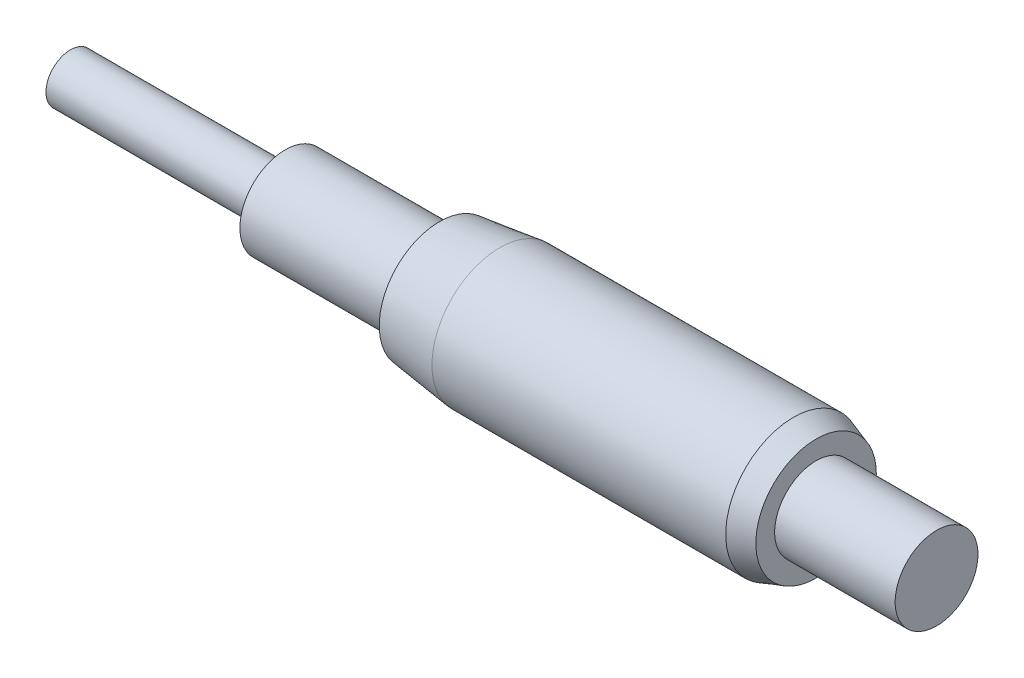
SolidWorks part; units mm, degrees
ref_plane "Front Plane" through (0, 0, 0) normal (0, 0, 1) x (1, 0, 0)
ref_plane "Top Plane" through (0, 0, 0) normal (0, 1, 0) x (1, 0, 0)
ref_plane "Right Plane" through (0, 0, 0) normal (1, 0, 0) x (0, 0, -1)
sketch "Sketch1" plane through (0, 0, 0) normal (0, 0, 1) x (1, 0, 0)
  line L0 (28.5, 3.25) -> (0, 3.25)
  line L1 (0, 3.25) -> (0, 0)
  line L2 (57, 9) -> (96, 9)
  line L3 (49, 8) -> (57, 9)
  line L4 (49, 6) -> (28.5, 6)
  line L5 (28.5, 6) -> (28.5, 3.25)
  line L7 (49, 8) -> (49, 6)
  line L8 (99, 5.5) -> (99, 8)
  line L9 (99, 8) -> (96, 9)
  line L10 (115, 0) -> (115, 5.5)
  line L11 (115, 5.5) -> (99, 5.5)
  line L12 (115, 0) -> (0, 0) construction
  line L13 (0, 0) -> (115, 0)
  dimension "D1" = 115
  dimension "D2" = 28.5
  dimension "D3" = 6
  dimension "D4" = 9
  dimension "D5" = 20.5
revolve "Revolve1" add sketch "Sketch1" angle 360 about L12
